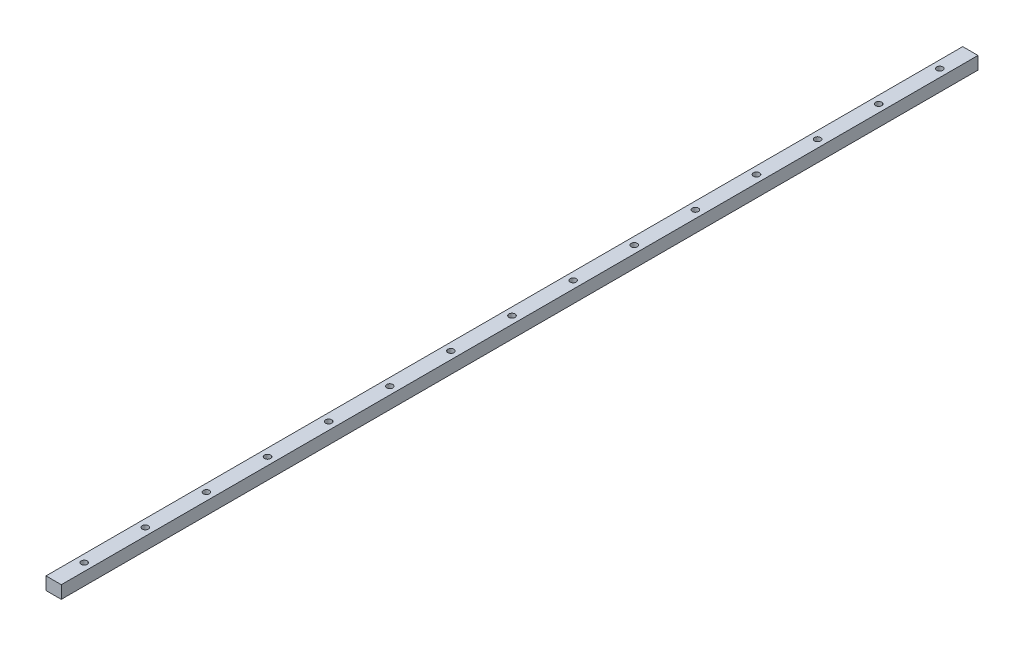
SolidWorks part; units mm, degrees
material "普通碳钢"
ref_plane "前视基准面" through (0, 0, 0) normal (0, 0, 1) x (1, 0, 0)
ref_plane "上视基准面" through (0, 0, 0) normal (0, 1, 0) x (1, 0, 0)
ref_plane "右视基准面" through (0, 0, 0) normal (1, 0, 0) x (0, 0, -1)
sketch "草图1" plane through (0, 0, 0) normal (0, 0, 1) x (1, 0, 0)
  line L1 (-7.5, 6.25) -> (7.5, 6.25)
  line L2 (-7.5, 6.25) -> (-7.5, -6.25)
  line L3 (-7.5, -6.25) -> (7.5, -6.25)
  line L4 (7.5, 6.25) -> (7.5, -6.25)
  line L5 (-7.5, 6.25) -> (7.5, -6.25) construction
  line L6 (-7.5, -6.25) -> (7.5, 6.25) construction
  point P0 (0, 0)
  dimension "D1" = 15
  dimension "D2" = 12.5
extrude "凸台-拉伸1" add sketch "草图1" along normal mid plane 900
sketch "草图2" plane through (0, 6.25, 0) normal (0, 1, 0) x (1, 0, 0)
  line L0 (0, -420) -> (0, -450) construction
  line L1 (7.5, -450) -> (-7.5, -450) construction
  circle A0 centre (0, -420) radius 3
  dimension "D2" = 6
  dimension "D1" = 30
extrude "切除-拉伸1" cut sketch "草图2" against normal blind 4.5
sketch "草图3" plane through (0, 6.25, 0) normal (0, 1, 0) x (1, 0, 0)
  circle A0 centre (0, -420) radius 2.25
  dimension "D1" = 4.5
extrude "切除-拉伸2" cut sketch "草图3" against normal through all
pattern_linear "阵列(线性)1" count 16 spacing 60 along (0, 0, -1) of "切除-拉伸1", "切除-拉伸2"
